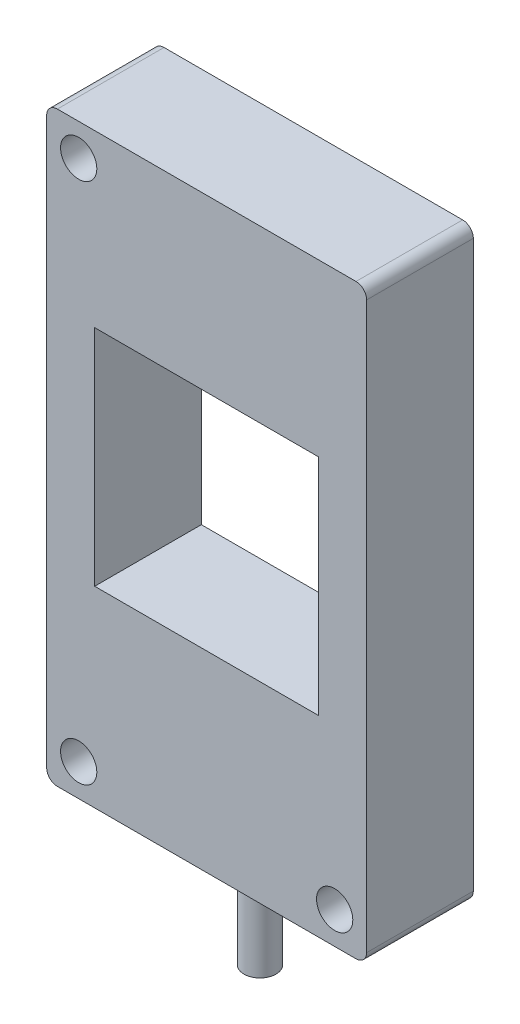
SolidWorks part; units mm, degrees
ref_plane "Front Plane" through (0, 0, 0) normal (0, 0, 1) x (1, 0, 0)
ref_plane "Top Plane" through (0, 0, 0) normal (0, 1, 0) x (1, 0, 0)
ref_plane "Right Plane" through (0, 0, 0) normal (1, 0, 0) x (0, 0, -1)
sketch "Sketch1" plane through (0, 0, 0) normal (0, 0, 1) x (1, 0, 0)
  line L1 (-15, 27.5) -> (15, 27.5)
  line L2 (-15, 27.5) -> (-15, -27.5)
  line L3 (-15, -27.5) -> (15, -27.5)
  line L4 (15, 27.5) -> (15, -27.5)
  line L5 (-15, 27.5) -> (15, -27.5) construction
  line L6 (-15, -27.5) -> (15, 27.5) construction
  point P0 (0, 0)
  dimension "D1" = 30
  dimension "D2" = 55
extrude "Boss-Extrude1" add sketch "Sketch1" along normal mid plane 10
sketch "Sketch2" plane through (0, 0, 5) normal (0, 0, 1) x (1, 0, 0)
  line L0 (15, 27.5) -> (-15, 27.5) construction
  line L1 (-10.5, 11.5) -> (10.5, 11.5)
  line L2 (-10.5, 11.5) -> (-10.5, -9.5)
  line L3 (-10.5, -9.5) -> (10.5, -9.5)
  line L4 (10.5, 11.5) -> (10.5, -9.5)
  line L5 (-10.5, 11.5) -> (10.5, -9.5) construction
  line L6 (-10.5, -9.5) -> (10.5, 11.5) construction
  point P0 (0, 1)
  dimension "D1" = 21
  dimension "D2" = 21
  dimension "D3" = 26.5
extrude "Cut-Extrude1" cut sketch "Sketch2" against normal through all
sketch "Sketch3" plane through (0, -27.5, 0) normal (0, -1, 0) x (1, 0, 0)
  circle A0 centre (0, 0) radius 1.5
  dimension "D1" = 3
extrude "Boss-Extrude2" add sketch "Sketch3" along normal blind 10
chamfer "Chamfer1" distance 1 angle 45 1 edges at (0, -27.5, 1.5)
fillet "Fillet1" radius 1 4 edges at (-15, -27.5, 0) (15, -27.5, 0) (15, 27.5, 0) (-15, 27.5, 0)
hole_wizard "Ø3.4 (3.4) Diameter Hole1" positions "Sketch5" profile "Sketch4" hole size "Ø3.4" standard "Gb" end condition through all
sketch "Sketch5" plane through (0, 0, 5) normal (0, 0, 1) x (1, 0, 0)
  line L0 (0, 0) -> (0, 20.0444) construction
  line L2 (-14, -27.5) -> (14, -27.5) construction
  line L3 (14, 27.5) -> (-14, 27.5) construction
  point P0 (-12, 24.5)
  point P2 (-12, -24.5)
  point P4 (12, -24.5)
  dimension "D1" = 24
  dimension "D2" = 3
  dimension "D3" = 3
sketch "Sketch4" plane through (-12, 24.5, 5) normal (1, 0, 0) x (0, -1, 0)
  line L0 (0, 0) -> (0, 10)
  line L1 (0, 10) -> (1.7, 10)
  line L2 (1.7, 10) -> (1.7, 0)
  line L5 (1.7, 0) -> (0, 0)
  line L11 (0, -6.35) -> (0, 107.95) construction
  dimension "通孔孔直径" = 3.4
  dimension "通孔孔深度" = 10
sketch "Sketch6" plane through (0, 0, 5) normal (0, 0, 1) x (1, 0, 0)
  line L0 (-10.5, 11.5) -> (-10.5, -9.5) construction
  line L1 (-10.5, -9.5) -> (10.5, -9.5) construction
  line L2 (10.5, -9.5) -> (10.5, 11.5) construction
  line L3 (10.5, 11.5) -> (-10.5, 11.5) construction
  circle A0 centre (0, 1) radius 10.5
